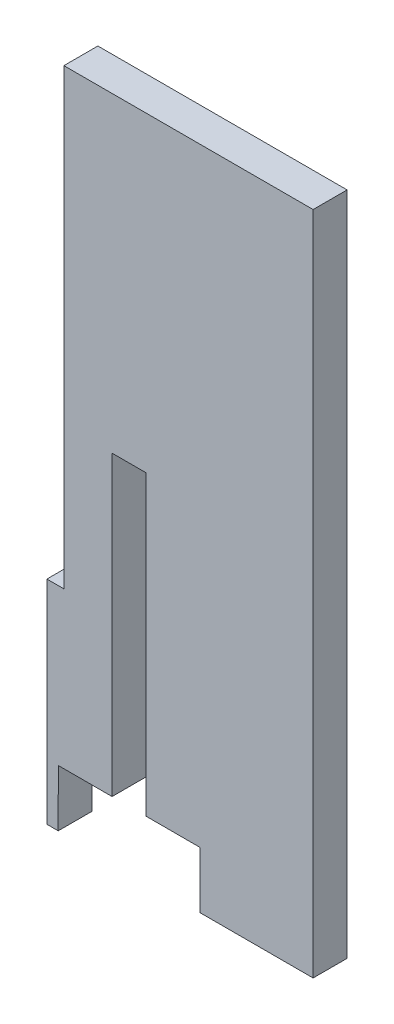
from build123d import *

# Parameters (mm, degrees)
BOSS_EXTRUDE1_DEPTH = 6
SKETCH3_W           = 6
SKETCH3_H           = 60
CUT_EXTRUDE1_DEPTH  = 10
CUT_EXTRUDE2_DEPTH  = 192.546823128


with BuildPart() as part:
    # Sketch1 → Boss-Extrude1 (new body)
    with BuildSketch(Plane.XY):
        Polygon((127.012699858, -33.445283653), (107.012699858, -33.445283653), (107.012699858, 84.054716347), (172.014505523, 84.054716347), (172.014505523, -33.445283653), (152.014505523, -33.445283653), (152.022415095, -23.465101408), (127.020625134, -23.445286794), align=None)
    extrude(amount=BOSS_EXTRUDE1_DEPTH)

    # Sketch3 → Cut-Extrude1 (cut)
    with BuildSketch(Plane(origin=(0, 0, 0), x_dir=(-1, 0, 0), z_dir=(0, 0, -1))):
        with Locations((-139.516482917, -0.945283653)):
            Rectangle(SKETCH3_W, SKETCH3_H)
    extrude(amount=-CUT_EXTRUDE1_DEPTH, mode=Mode.SUBTRACT)

    # Sketch4 → Cut-Extrude2 (cut, through all)
    with BuildSketch(Plane.XY.offset(6)):
        Polygon((125.012699858, -36.580409203), (107.012699858, -36.580409203), (107.012699858, 84.054716347), (128.012699858, 84.054716347), (128.012699858, 4.054716347), (125.012699858, 4.054716347), align=None)
    extrude(amount=-CUT_EXTRUDE2_DEPTH, mode=Mode.SUBTRACT)


solid = part.part
